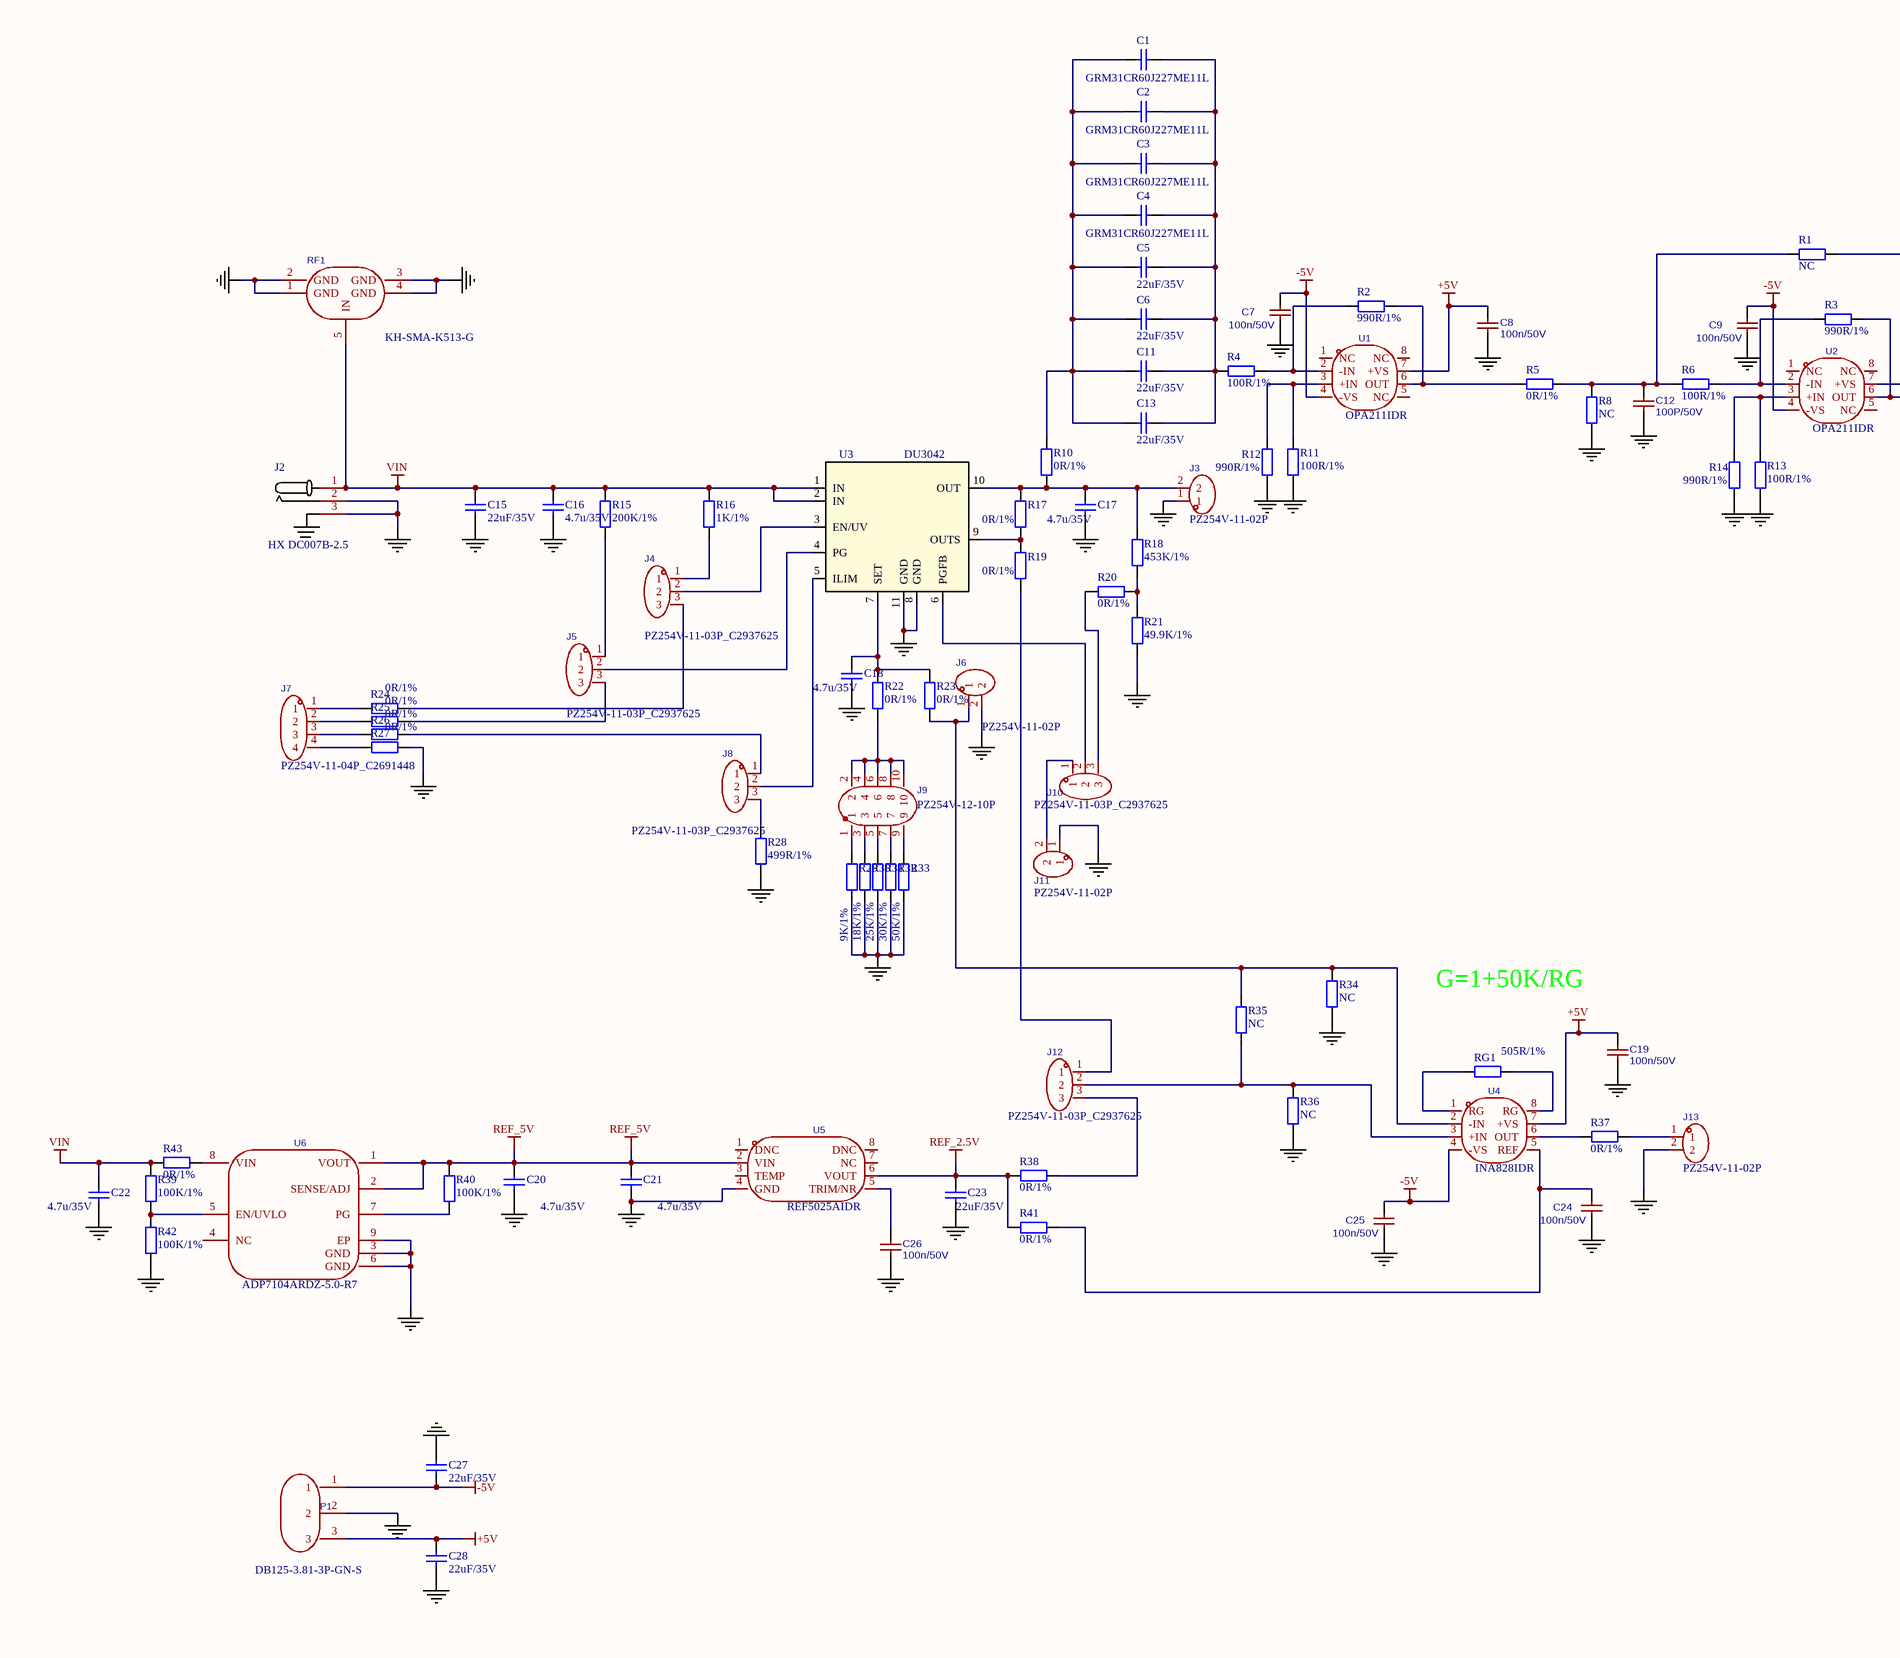
[diagram p0: MISC75514-12.SchDoc, left]
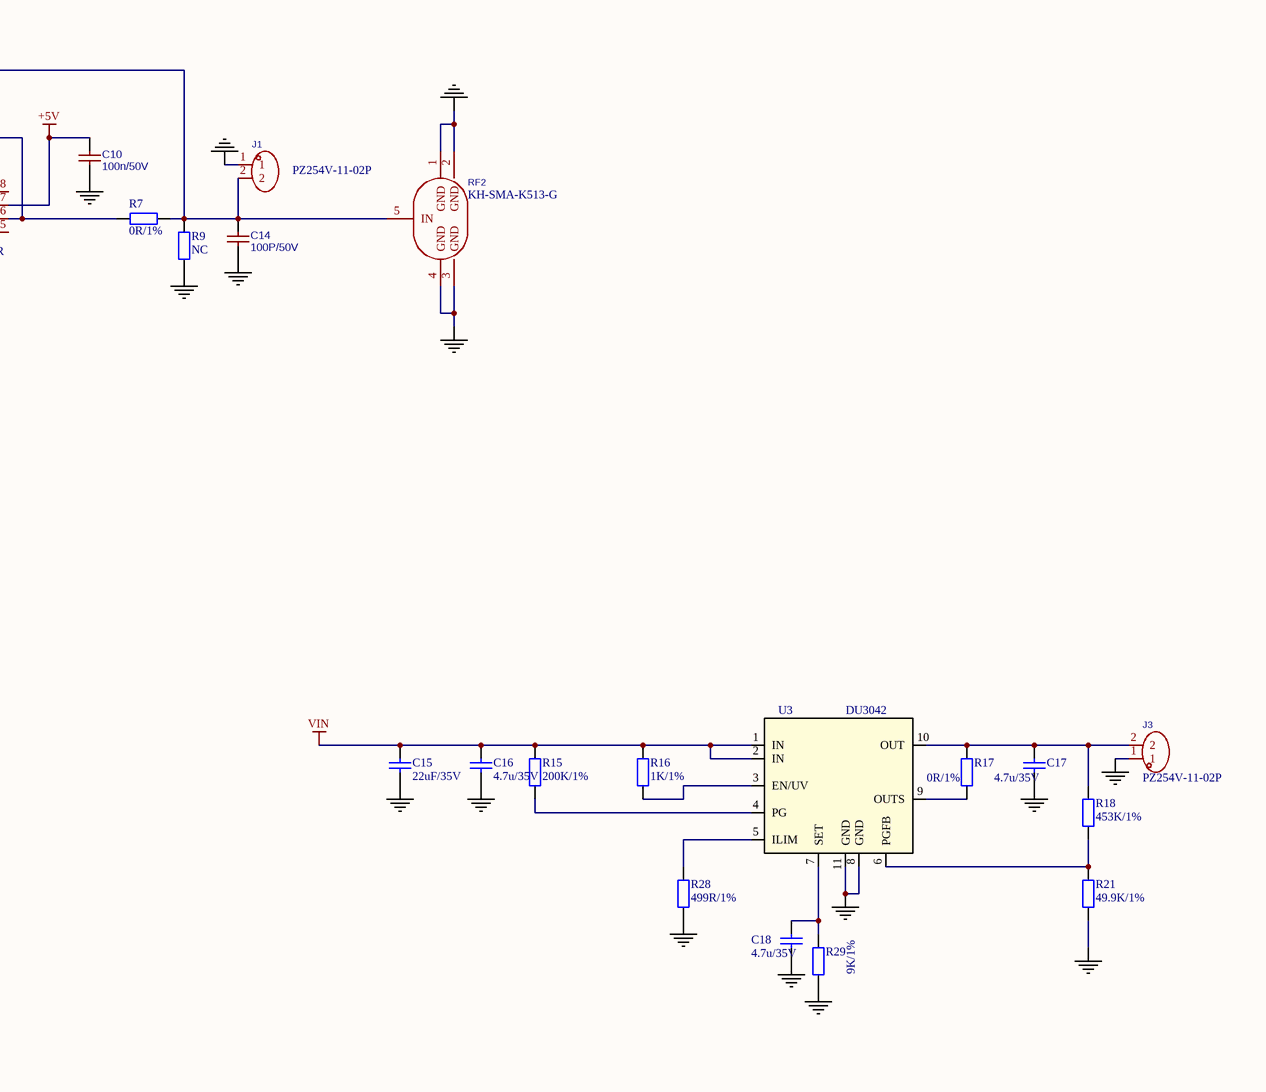
[diagram p1: MISC75514-12.SchDoc, right]
# Altium project MISC75514-7.PrjPCB
1 sheet, 107 parts. Net scope: global (net labels, ports and power ports of the same name join across sheets).
Board file: MISC75514.PcbDoc

## Sheet MISC75514-12.SchDoc
size A1

### Parts
(Parts that share a designator on the sheet are numbered #1, #2 ... from top to bottom, then left to right.)
C1  GRM31CR60J227ME11L  [C1206]
C2  GRM31CR60J227ME11L  [C1206]
C3  GRM31CR60J227ME11L  [C1206]
C4  GRM31CR60J227ME11L  [C1206]
C5  22uF/35V  [C1206]
C6  22uF/35V  [C1206]
C7  100n/50V  [C0603]
C8  100n/50V  [C0603]
C9  100n/50V  [C0603]
C10  100n/50V  [C0603]
C11  22uF/35V  [C1206]
C12  100P/50V  [C0603]
C13  22uF/35V  [C1206]
C14  100P/50V  [C0603]
C15#1  22uF/35V  [C1206]
C15#2  22uF/35V  [C1206]
C16#1  4.7u/35V  [C0805]
C16#2  4.7u/35V  [C0805]
C17#1  4.7u/35V  [C0805]
C17#2  4.7u/35V  [C0805]
C18#1  4.7u/35V  [C0805]
C18#2  4.7u/35V  [C0805]
C19  100n/50V  [C0603]
C20  4.7u/35V  [C0805]
C21  4.7u/35V  [C0805]
C22  4.7u/35V  [C0805]
C23  22uF/35V  [C1206]
C24  100n/50V  [C0603]
C25  100n/50V  [C0603]
C26  100n/50V  [C0603]
C27  22uF/35V  [C1206]
C28  22uF/35V  [C1206]
J1  PZ254V-11-02P  [HDR-TH_2P-P2.54-V-M]
J2  HX DC007B-2.5  [DC-IN-TH_HX-DC007B-2.5]
J3#1  PZ254V-11-02P  [HDR-TH_2P-P2.54-V-M]
J3#2  PZ254V-11-02P  [HDR-TH_2P-P2.54-V-M]
J4  PZ254V-11-03P_C2937625  [HDR-TH_3P-P2.54-V-M]
J5  PZ254V-11-03P_C2937625  [HDR-TH_3P-P2.54-V-M]
J6  PZ254V-11-02P  [HDR-TH_2P-P2.54-V-M]
J7  PZ254V-11-04P_C2691448  [HDR-TH_4P-P2.54-V-M]
J8  PZ254V-11-03P_C2937625  [HDR-TH_3P-P2.54-V-M]
J9  PZ254V-12-10P  [HDR-TH_10P-P2.54-V-M-R2-C5-S2.54]
J10  PZ254V-11-03P_C2937625  [HDR-TH_3P-P2.54-V-M]
J11  PZ254V-11-02P  [HDR-TH_2P-P2.54-V-M]
J12  PZ254V-11-03P_C2937625  [HDR-TH_3P-P2.54-V-M]
J13  PZ254V-11-02P  [HDR-TH_2P-P2.54-V-M]
P1  DB125-3.81-3P-GN-S  [CONN-TH_3P-P3.81_L7.4-W11.4]
R1  NC  [R0603]
R2  990R/1%  [R0603]
R3  990R/1%  [R0603]
R4  100R/1%  [R0603]
R5  0R/1%  [R0603]
R6  100R/1%  [R0603]
R7  0R/1%  [R0603]
R8  NC  [R0603]
R9  NC  [R0603]
R10  0R/1%  [R0603]
R11  100R/1%  [R0603]
R12  990R/1%  [R0603]
R13  100R/1%  [R0603]
R14  990R/1%  [R0603]
R15#1  200K/1%  [R0603]
R15#2  200K/1%  [R0603]
R16#1  1K/1%  [R0603]
R16#2  1K/1%  [R0603]
R17#1  0R/1%  [R0603]
R17#2  0R/1%  [R0603]
R18#1  453K/1%  [R0603]
R18#2  453K/1%  [R0603]
R19  0R/1%  [R0603]
R20  0R/1%  [R0603]
R21#1  49.9K/1%  [R0603]
R21#2  49.9K/1%  [R0603]
R22  0R/1%  [R0603]
R23  0R/1%  [R0603]
R24  0R/1%  [R0603]
R25  0R/1%  [R0603]
R26  0R/1%  [R0603]
R27  0R/1%  [R0603]
R28#1  499R/1%  [R0603]
R28#2  499R/1%  [R0603]
R29#1  9K/1%  [R0603]
R29#2  9K/1%  [R0603]
R30  18K/1%  [R0603]
R31  25K/1%  [R0603]
R32  30K/1%  [R0603]
R33  50K/1%  [R0603]
R34  NC  [R0603]
R35  NC  [R0603]
R36  NC  [R0603]
R37  0R/1%  [R0603]
R38  0R/1%  [R0603]
R39  100K/1%  [R0603]
R40  100K/1%  [R0603]
R41  0R/1%  [R0603]
R42  100K/1%  [R0603]
R43  0R/1%  [R0603]
RF1  KH-SMA-K513-G  [ANT-TH_KH-SMA-K513-G]
RF2  KH-SMA-K513-G  [ANT-TH_KH-SMA-K513-G]
RG1  505R/1%  [R0603]
U1  OPA211IDR  [SOIC-8_L5.0-W4.0-P1.27-LS6.0-BL]
U2  OPA211IDR  [SOIC-8_L5.0-W4.0-P1.27-LS6.0-BL]
U3#1  DU3042  [WSON-10_L3.0-W3.0-P0.50-BL-EP]
U3#2  DU3042  [WSON-10_L3.0-W3.0-P0.50-BL-EP]
U4  INA828IDR  [SOIC-8_L5.0-W4.0-P1.27-LS6.0-BL]
U5  REF5025AIDR  [SOIC-8_L5.0-W4.0-P1.27-LS6.0-BL]
U6  ADP7104ARDZ-5.0-R7  [SOIC-8_L4.9-W3.9-P1.27-LS6.0-BL-EP]

### Nets
+5V: C8.1 C10.1 C19.1 C28.2 P1.3 U1.7(+VS) U2.7(+VS) U4.7(+VS)
-5V: C7.1 C9.1 C25.1 C27.2 P1.1 U1.4(-VS) U2.4(-VS) U4.4(-VS)
GND: C7.2 C8.2 C9.2 C10.2 C12.2 C14.2 C15#1.1 C15#2.1 C16#1.1 C16#2.1 C17#1.1 C17#2.1 C18#1.1 C18#2.1 C19.2 C20.1 C21.1 C22.1 C23.2 C24.2 C25.2 C26.2 C27.1 C28.1 J1.1 J2.2 J2.3 J3#1.1 J3#2.1 J6.2 J11.1 J13.2 P1.2 R8.1 R9.1 R11.1 R12.1 R13.1 R14.1 R21#1.2 R21#2.2 R27.1 R28#1.1 R28#2.1 R29#1.1 R29#2.1 R30.1 R31.1 R32.1 R33.1 R34.2 R36.2 R42.1 RF1.1(GND) RF1.2(GND) RF1.3(GND) RF1.4(GND) RF2.1(GND) RF2.2(GND) RF2.3(GND) RF2.4(GND) U3#1.8(GND) U3#1.11(GND) U3#2.8(GND) U3#2.11(GND) U5.4(GND) U6.3(GND) U6.6(GND) U6.9(EP)
REF_2.5V: C23.1 R38.1 R41.1 U5.6(VOUT)
REF_5V: C20.2 C21.2 R40.2 U5.2(VIN) U6.1(VOUT) U6.2(SENSE/ADJ)
VIN: C15#1.2 C15#2.2 C16#1.2 C16#2.2 C22.2 J2.1 R15#1.2 R15#2.2 R16#1.2 R16#2.2 R39.2 R43.1 RF1.5(IN) U3#1.1(IN) U3#1.2(IN) U3#2.1(IN) U3#2.2(IN)
NetC1_1: C1.1 C2.1 C3.1 C4.1 C5.1 C6.1 C11.1 C13.1 R4.1
NetC1_2: C1.2 C2.2 C3.2 C4.2 C5.2 C6.2 C11.2 C13.2 R10.1
NetC12_1: C12.1 R1.2 R5.2 R6.1 R8.2
NetC14_1: C14.1 J1.2 R1.1 R7.2 R9.2 RF2.5(IN)
NetC17#1_2: C17#1.2 J3#1.2 R10.2 R17#1.1 R18#1.1 U3#1.10(OUT)
NetC17#2_2: C17#2.2 J3#2.2 R17#2.1 R18#2.1 U3#2.10(OUT)
NetC18#1_2: C18#1.2 R22.1 R23.1 U3#1.7(SET)
NetC18#2_2: C18#2.2 R29#2.2 U3#2.7(SET)
NetC24_1: C24.1 R41.2 U4.5(REF)
NetC26_1: C26.1 U5.5(TRIM/NR)
NetJ4_1: J4.1 R16#1.1
NetJ4_2: J4.2 U3#1.3(EN/UV)
NetJ4_3: J4.3 R24.1
NetJ5_1: J5.1 R15#1.1
NetJ5_2: J5.2 U3#1.4(PG)
NetJ5_3: J5.3 R25.1
NetJ6_1: J6.1 R23.2 R34.1 R35.1 U4.2(-IN)
NetJ7_1: J7.1 R24.2
NetJ7_2: J7.2 R25.2
NetJ7_3: J7.3 R26.2
NetJ7_4: J7.4 R27.2
NetJ8_1: J8.1 R26.1
NetJ8_2: J8.2 U3#1.5(ILIM)
NetJ8_3: J8.3 R28#1.2
NetJ9_1: J9.1 R29#1.2
NetJ9_2: J9.2 J9.4 J9.6 J9.8 J9.10 R22.2
NetJ9_3: J9.3 R30.2
NetJ9_5: J9.5 R31.2
NetJ9_7: J9.7 R32.2
NetJ9_9: J9.9 R33.2
NetJ10_1: J10.1 J11.2
NetJ10_2: J10.2 U3#1.6(PGFB)
NetJ10_3: J10.3 R20.1
NetJ12_1: J12.1 R19.2
NetJ12_2: J12.2 R35.2 R36.1 U4.3(+IN)
NetJ12_3: J12.3 R38.2
NetJ13_1: J13.1 R37.2
NetR2_1: R2.1 R5.1 U1.6(OUT)
NetR2_2: R2.2 R4.2 U1.2(-IN)
NetR3_1: R3.1 R7.1 U2.6(OUT)
NetR3_2: R3.2 R6.2 U2.2(-IN)
NetR11_2: R11.2 R12.2 U1.3(+IN)
NetR13_2: R13.2 R14.2 U2.3(+IN)
NetR15#2_1: R15#2.1 U3#2.4(PG)
NetR16#2_1: R16#2.1 U3#2.3(EN/UV)
NetR17#1_2: R17#1.2 R19.1 U3#1.9(OUTS)
NetR17#2_2: R17#2.2 U3#2.9(OUTS)
NetR18#1_2: R18#1.2 R20.2 R21#1.1
NetR18#2_2: R18#2.2 R21#2.1 U3#2.6(PGFB)
NetR28#2_2: R28#2.2 U3#2.5(ILIM)
NetR37_1: R37.1 U4.6(OUT)
NetR39_1: R39.1 R42.2 U6.5(EN/UVLO)
NetR40_1: R40.1 U6.7(PG)
NetR43_2: R43.2 U6.8(VIN)
NetRG1_1: RG1.1 U4.8(RG)
NetRG1_2: RG1.2 U4.1(RG)

Not connected (* = marked no-connect by the designer): U1 1(NC) 5(NC) 8(NC); U2 1(NC) 5(NC) 8(NC); U5 1(DNC) 3(TEMP) 7(NC) 8(DNC); U6 4(NC)

### Notes on the sheet
- G=1+50K/RG

### Library data of the parts
C1-C6 C11 C13 C15#1 C15#2 C16#1 C16#2 C17#1 C17#2 C18#1 C18#2 C20-C23 C27 C28 = C: SMD capacitor; BOM名称: Non-polar SMD capacitor
C7-C10 C12 C14 C19 C24-C26 = 1uF: Manufacturer Part: CL10A105KB8NNNC; nameAlias: Value; Supplier: LCSC; Supplier Part: C15849; JLCPCB Part Class: Basic Part; spicePre: C; spiceSymbolName: CL10A105KB8NNNC
J2 = HX DC007B-2.5: Manufacturer: hanxia(韩下); Add into BOM: yes; Connector Type: DC power jack; Inside Contact Diameter: 2.5mm; Outside Contact Diameter: 6.4mm; Current Rating (Max): 7A; Voltage Rating (Max): 20V; Name: HX DC007B-2.5; Symbol: HX DC007B-2.5; Device: HX DC007B-2.5; Supplier: LCSC; Supplier Part: C19189083; Manufacturer Part: HX DC007B-2.5; LCSC Part Name: DC电源插座 内径:2.5mm 外径:6.4mm; Supplier Footprint: 插件; Datasheet: https://atta.szlcsc.com/upload/public/pdf/source/20231103/814B3421283469BAAEFFF9B7A53EC0CB.pdf; Convert to PCB: yes; Mounting Style: Right angle THT; Operating Temperature Range: -25℃~+70℃
P1 = WJ124-3.81-3P: Symbol: WJ124-3.81-3P
R1-R14 R15#1 R15#2 R16#1 R16#2 R17#1 R17#2 R18#1 R18#2 R19 R20 R21#1 R21#2 R22-R27 R28#1 R28#2 R29#1 R29#2 R30-R43 RG1 = R: SMD resistor; BOM名称: SMD resistor
U1 U2 = INA828IDR: Symbol: INA828IDR
U3#1 U3#2 = DAC53202RTER: No Description Available; Mfr_Name: Texas Instruments; Type: Data Acquisition; RefDes: RefDes
J1 J3#1 J3#2 J6 J11 J13 = PZ254V-11-02P: Symbol: PZ254V-11-02P
J4 J5 J8 J10 J12 = PZ254V-11-03P_C2937625: Symbol: PZ254V-11-03P_C2937625
J7 = PZ254V-11-04P_C2691448: Symbol: PZ254V-11-04P_C2691448
J9 = PZ254V-12-10P: Symbol: PZ254V-12-10P
RF1 RF2 = KH-SMA-K513-G: Symbol: KH-SMA-K513-G
U4 = INA828IDR: Symbol: INA828IDR
U5 = REF5025AIDR: Symbol: REF5025AIDR
U6 = ADP7104ARDZ-5.0-R7: Symbol: ADP7104ARDZ-5.0-R7